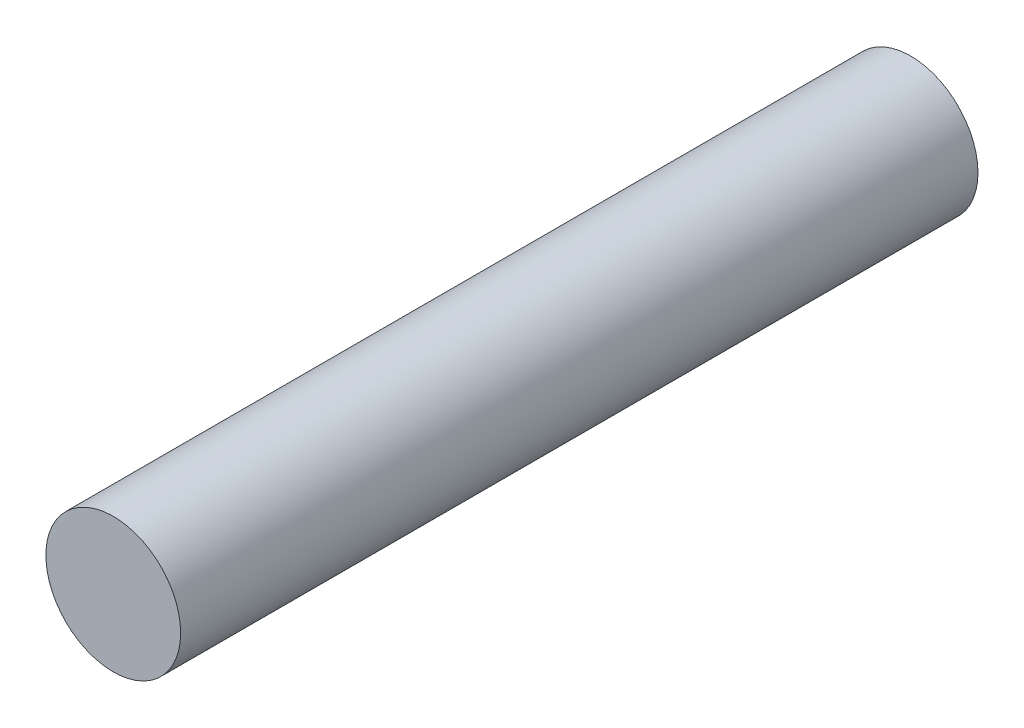
from build123d import *

# Parameters (mm, degrees)
SKETCH_1_R      = 6
EXTRUDE_1_DEPTH = 35.5


with BuildPart() as part:
    # 草图1 → 凸台-拉伸1 (new, symmetric)
    with BuildSketch(Plane.XY):
        Circle(SKETCH_1_R)
    extrude(amount=EXTRUDE_1_DEPTH, both=True)


solid = part.part
